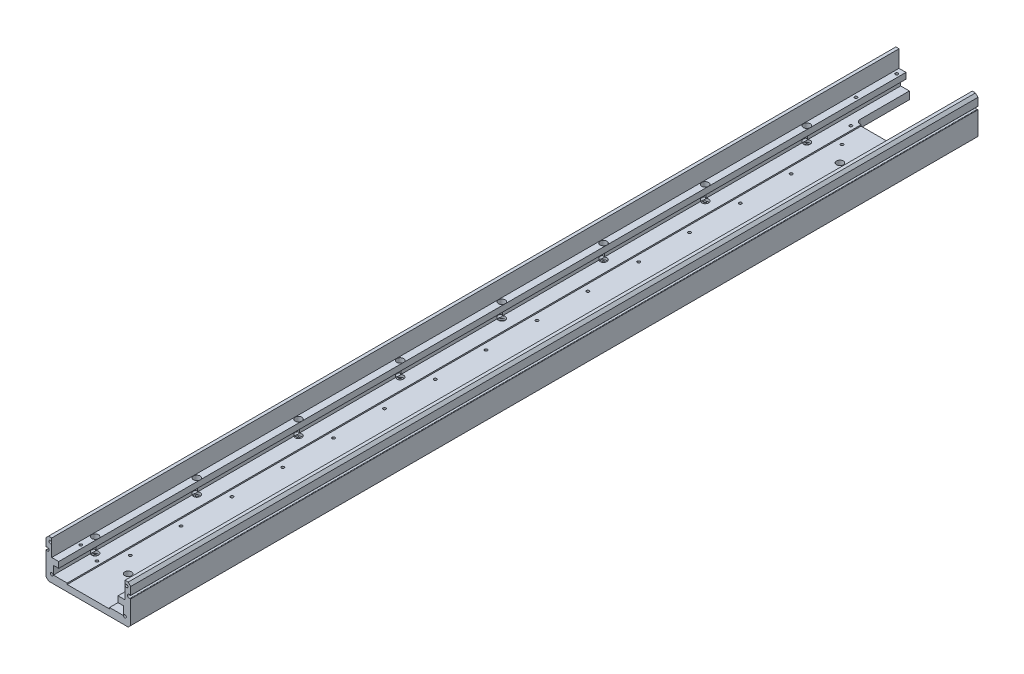
from build123d import *

# Parameters (mm, degrees)
SKETCH_1_W                  = 100
SKETCH_1_H                  = 46
EXTRUDE_1_DEPTH             = 500
CHAMFER_1_SIZE              = 3
CUT_EXTRUDE_1_DEPTH         = 504.019880323
CUT_EXTRUDE_1_DEPTH_BACK    = 504.019880323
CUT_EXTRUDE_2_DEPTH         = 504.019880323
CUT_EXTRUDE_2_DEPTH_BACK    = 504.019880323
SKETCH_3_R                  = 1.6
CUT_EXTRUDE_3_DEPTH         = 504.019880323
CUT_EXTRUDE_3_DEPTH_BACK    = 504.019880323
SKETCH_4_R                  = 2
SKETCH_5_W                  = 62
SKETCH_5_H                  = 63
CUT_EXTRUDE_4_DEPTH         = 505.594887013
HOLE_WIZARD_M4_1_AT_2_COUNT = 2
HOLE_WIZARD_M4_1_AT_2_PITCH = 32.053431954
HOLE_WIZARD_M4_1_AT_3_COUNT = 2
HOLE_WIZARD_M4_1_AT_3_PITCH = 93.77858231
HOLE_WIZARD_M4_1_AT_4_COUNT = 2
HOLE_WIZARD_M4_1_AT_4_PITCH = 86.3
FILLET_1_R                  = 5
HOLE_WIZARD_M4_2_REACH      = 505.166
HOLE_WIZARD_M4_2_BORE_R     = 1.65
FILLET_2_R                  = 0.35
HOLE_WIZARD_M4_3_D          = 3.3
PATTERN_LINEAR_1_COUNT      = 15
PATTERN_LINEAR_1_PITCH      = 60
HOLE_WIZARD_2_D             = 4.5
HOLE_WIZARD_2_CBORE_D       = 7.99
HOLE_WIZARD_2_CBORE_DEPTH   = 20
PATTERN_LINEAR_2_COUNT      = 8
PATTERN_LINEAR_2_PITCH      = 120
HOLE_WIZARD_M4_4_D          = 3.3
PATTERN_LINEAR_4_COUNT      = 2
PATTERN_LINEAR_4_PITCH      = 890
SKETCH_25_R                 = 4
CUT_EXTRUDE_6_DEPTH         = 10


with BuildPart() as part:
    # 草图1 → 凸台-拉伸1 (new, symmetric)
    with BuildSketch(Plane.XY):
        Rectangle(SKETCH_1_W, SKETCH_1_H)
    extrude(amount=EXTRUDE_1_DEPTH, both=True)

    # 倒角1
    chamfer_1_edges = [part.edges().sort_by_distance(p)[0] for p in [
        (50, -23, 0),
        (-50, -23, 0),
        (-50, 23, 0),
        (50, 23, 0),
    ]]
    chamfer(chamfer_1_edges, length=CHAMFER_1_SIZE)

    # 草图2 → 切除-拉伸1 (cut, two sides: drawn at the far end of the back side and taken through both)
    with BuildSketch(Plane.XY.offset(-CUT_EXTRUDE_1_DEPTH_BACK)):
        Polygon((43.25, 23), (-43.25, 23), (-43.25, 3), (-35, 3), (-35, -4), (-41.25, -4), (-41.25, -14), (-25, -14), (-25, -15.5), (25, -15.5), (25, -14), (41.25, -14), (41.25, -4), (35, -4), (35, 3), (43.25, 3), align=None)
    extrude(amount=CUT_EXTRUDE_1_DEPTH + CUT_EXTRUDE_1_DEPTH_BACK, mode=Mode.SUBTRACT)

    # 草图3 → 切除-拉伸2 (cut, two sides: drawn at the far end of the back side and taken through both)
    with BuildSketch(Plane.XY.offset(-CUT_EXTRUDE_2_DEPTH_BACK)):
        with Locations((-43.15, -14)):
            Circle(SKETCH_3_R)
        with Locations((-45, 18)):
            Circle(SKETCH_3_R)
        with Locations(Location((43.15, -14, 0), (0, 0, 180))):
            Circle(SKETCH_3_R)
        with Locations(Location((45, 18, 0), (0, 0, 180))):
            Circle(SKETCH_3_R)
    extrude(amount=CUT_EXTRUDE_2_DEPTH + CUT_EXTRUDE_2_DEPTH_BACK, mode=Mode.SUBTRACT)

    # 草图4 → 切除-拉伸3 (cut, two sides: drawn at the far end of the back side and taken through both)
    with BuildSketch(Plane.XY.offset(-CUT_EXTRUDE_3_DEPTH_BACK)):
        with Locations((-48.2, 9.1)):
            Circle(SKETCH_4_R)
        with Locations((48.2, 9.1)):
            Circle(SKETCH_4_R)
    extrude(amount=CUT_EXTRUDE_3_DEPTH + CUT_EXTRUDE_3_DEPTH_BACK, mode=Mode.SUBTRACT)

    # 草图5 → 切除-拉伸4 (cut, through all)
    with BuildSketch(Plane.XZ.offset(23)):
        with Locations((0, -468.5)):
            Rectangle(SKETCH_5_W, SKETCH_5_H)
    extrude(amount=-CUT_EXTRUDE_4_DEPTH, mode=Mode.SUBTRACT)

    # 草图8 → M4 螺纹孔1 (revolve, cut)
    with BuildSketch(Plane(origin=(-43.15, -14, 500), x_dir=(0, -1, 0), z_dir=(1, 0, 0))):
        Polygon((0, 0), (0, 12.991420021), (1.65, 12), (1.65, 0), align=None)
    hole_wizard_m4_1 = revolve(axis=Axis((-43.15, -14, 506.35), (0, 0, -1)), mode=Mode.SUBTRACT)

    # M4 螺纹孔1 at 2: M4 螺纹孔1 ×2
    with Locations(*[Vector(-0.05771612857810949, 0.9983330348645962, 0) * (i * HOLE_WIZARD_M4_1_AT_2_PITCH) for i in range(1, HOLE_WIZARD_M4_1_AT_2_COUNT)]):
        add(hole_wizard_m4_1, mode=Mode.SUBTRACT)

    # M4 螺纹孔1 at 3: M4 螺纹孔1 ×2
    with Locations(*[Vector(0.9399800874465586, 0.34122930003732144, 0) * (i * HOLE_WIZARD_M4_1_AT_3_PITCH) for i in range(1, HOLE_WIZARD_M4_1_AT_3_COUNT)]):
        add(hole_wizard_m4_1, mode=Mode.SUBTRACT)

    # M4 螺纹孔1 at 4: M4 螺纹孔1 ×2
    with Locations(*[(i * HOLE_WIZARD_M4_1_AT_4_PITCH, 0, 0) for i in range(1, HOLE_WIZARD_M4_1_AT_4_COUNT)]):
        add(hole_wizard_m4_1, mode=Mode.SUBTRACT)

    # 镜向3: M4 螺纹孔1 across plane
    add(hole_wizard_m4_1.mirror(Plane.XY), mode=Mode.SUBTRACT)

    # 镜向3 copy 1 sketch → 镜向3 copy 1 (revolve, cut)
    with BuildSketch(Plane(origin=(-45, 18, -500), x_dir=(0, -1, 0), z_dir=(1, 0, 0))):
        Polygon((0, 0), (0, -12.991420021), (1.65, -12), (1.65, 0), align=None)
    revolve(axis=Axis((-45, 18, -506.35), (0, 0, -1)), mode=Mode.SUBTRACT)

    # 镜向3 copy 2 sketch → 镜向3 copy 2 (revolve, cut)
    with BuildSketch(Plane(origin=(45, 18, -500), x_dir=(0, -1, 0), z_dir=(1, 0, 0))):
        Polygon((0, 0), (0, -12.991420021), (1.65, -12), (1.65, 0), align=None)
    revolve(axis=Axis((45, 18, -506.35), (0, 0, -1)), mode=Mode.SUBTRACT)

    # 镜向3 copy 3 sketch → 镜向3 copy 3 (revolve, cut)
    with BuildSketch(Plane(origin=(43.15, -14, -500), x_dir=(0, -1, 0), z_dir=(1, 0, 0))):
        Polygon((0, 0), (0, -12.991420021), (1.65, -12), (1.65, 0), align=None)
    revolve(axis=Axis((43.15, -14, -506.35), (0, 0, -1)), mode=Mode.SUBTRACT)

    # 圆角1
    fillet_1_edges = [part.edges().sort_by_distance(p)[0] for p in [
        (31, -18.5, -437),
        (-31, -18.5, -437),
    ]]
    fillet(fillet_1_edges, radius=FILLET_1_R)

    # M4 螺纹孔2 bore → M4 螺纹孔2 (cut, up to next)
    with BuildSketch(Plane(origin=(0, 3, 0), x_dir=(1, 0, 0), z_dir=(0, 1, 0)), mode=Mode.PRIVATE) as hole_wizard_m4_2_sk1:
        with Locations((-39, 493)):
            Circle(HOLE_WIZARD_M4_2_BORE_R)
    hole_wizard_m4_2_tool1 = extrude(hole_wizard_m4_2_sk1.sketch, amount=-HOLE_WIZARD_M4_2_REACH, mode=Mode.PRIVATE) & part.part
    # M4 螺纹孔2 bore → M4 螺纹孔2 (cut, up to next)
    with BuildSketch(Plane(origin=(0, 3, 0), x_dir=(1, 0, 0), z_dir=(0, 1, 0)), mode=Mode.PRIVATE) as hole_wizard_m4_2_sk2:
        with Locations((-39, 445)):
            Circle(HOLE_WIZARD_M4_2_BORE_R)
    hole_wizard_m4_2_tool2 = extrude(hole_wizard_m4_2_sk2.sketch, amount=-HOLE_WIZARD_M4_2_REACH, mode=Mode.PRIVATE) & part.part
    # M4 螺纹孔2 bore → M4 螺纹孔2 (cut, up to next)
    with BuildSketch(Plane(origin=(0, 3, 0), x_dir=(1, 0, 0), z_dir=(0, 1, 0)), mode=Mode.PRIVATE) as hole_wizard_m4_2_sk3:
        with Locations((-39, -470)):
            Circle(HOLE_WIZARD_M4_2_BORE_R)
    hole_wizard_m4_2_tool3 = extrude(hole_wizard_m4_2_sk3.sketch, amount=-HOLE_WIZARD_M4_2_REACH, mode=Mode.PRIVATE) & part.part
    hole_wizard_m4_2_1 = hole_wizard_m4_2_tool1.solids().sort_by_distance((-39, 3, -493))[0]
    add(hole_wizard_m4_2_1, mode=Mode.SUBTRACT)
    hole_wizard_m4_2_2 = hole_wizard_m4_2_tool2.solids().sort_by_distance((-39, 3, -445))[0]
    add(hole_wizard_m4_2_2, mode=Mode.SUBTRACT)
    hole_wizard_m4_2_3 = hole_wizard_m4_2_tool3.solids().sort_by_distance((-39, 3, 470))[0]
    add(hole_wizard_m4_2_3, mode=Mode.SUBTRACT)
    hole_wizard_m4_2 = hole_wizard_m4_2_1 + hole_wizard_m4_2_2 + hole_wizard_m4_2_3  # M4 螺纹孔2 as one shape, for the pattern or mirror that repeats it

    # 镜向4: M4 螺纹孔2 across plane
    add(hole_wizard_m4_2.mirror(Plane(origin=(0, 0, 0), x_dir=(0, 0, 1), z_dir=(1, 0, 0))), mode=Mode.SUBTRACT)

    # 圆角2
    fillet_2_edges = [part.edges().sort_by_distance(p)[0] for p in [
        (-50, 9.971779789, 0),
        (-50, 8.228220211, 0),
        (50, 8.228220211, 0),
        (50, 9.971779789, 0),
    ]]
    fillet(fillet_2_edges, radius=FILLET_2_R)

    # M4 螺纹孔3 (through all)
    with Locations(Plane(origin=(0, -15.5, 0), x_dir=(1, 0, 0), z_dir=(0, 1, 0))):
        with Locations((17.5, 407), (-17.5, 407)):
            hole_wizard_m4_3 = Hole(HOLE_WIZARD_M4_3_D / 2)

    # 阵列(线性)1: M4 螺纹孔3 ×15
    with Locations(*[(0, 0, i * PATTERN_LINEAR_1_PITCH) for i in range(1, PATTERN_LINEAR_1_COUNT)]):
        add(hole_wizard_m4_3, mode=Mode.SUBTRACT)

    # 打孔尺寸(%根据)开槽圆柱头螺钉的类型2 (through all)
    with Locations(Plane(origin=(0, 3, 0), x_dir=(1, 0, 0), z_dir=(0, 1, 0))):
        with Locations((-39, 387), (39, 387)):
            hole_wizard_2 = CounterBoreHole(HOLE_WIZARD_2_D / 2, HOLE_WIZARD_2_CBORE_D / 2, HOLE_WIZARD_2_CBORE_DEPTH)

    # 阵列(线性)2: 打孔尺寸(%根据)开槽圆柱头螺钉的类型2 ×8
    with Locations(*[(0, 0, i * PATTERN_LINEAR_2_PITCH) for i in range(1, PATTERN_LINEAR_2_COUNT)]):
        add(hole_wizard_2, mode=Mode.SUBTRACT)

    # M4 螺纹孔4 (through all)
    with Locations(Plane(origin=(0, -14, 0), x_dir=(1, 0, 0), z_dir=(0, 1, 0))):
        with Locations((30, 430), (-30, 430)):
            hole_wizard_m4_4 = Hole(HOLE_WIZARD_M4_4_D / 2)

    # 阵列(线性)4: M4 螺纹孔4 ×2
    with Locations(*[(0, 0, i * PATTERN_LINEAR_4_PITCH) for i in range(1, PATTERN_LINEAR_4_COUNT)]):
        add(hole_wizard_m4_4, mode=Mode.SUBTRACT)

    # 草图25 → 切除-拉伸6 (cut)
    with BuildSketch(Plane(origin=(0, -15.5, 0), x_dir=(1, 0, 0), z_dir=(0, 1, 0))):
        with Locations(Location((0, -453, 0), (0, 0, 180))):
            Circle(SKETCH_25_R)
        with Locations(Location((0, 387, 0), (0, 0, 180))):
            Circle(SKETCH_25_R)
    extrude(amount=-CUT_EXTRUDE_6_DEPTH, mode=Mode.SUBTRACT)


solid = part.part
